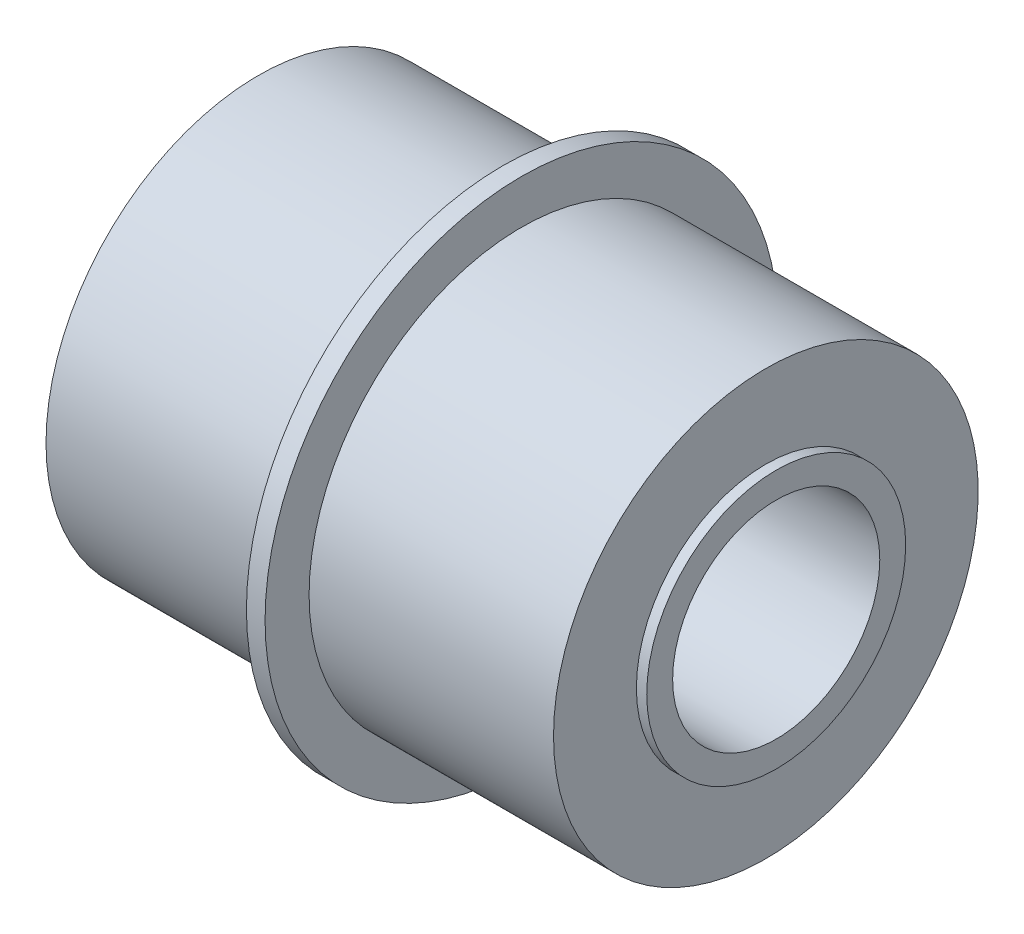
SolidWorks part; units mm, degrees
ref_plane "前视基准面" through (0, 0, 0) normal (0, 0, 1) x (1, 0, 0)
ref_plane "上视基准面" through (0, 0, 0) normal (0, 1, 0) x (1, 0, 0)
ref_plane "右视基准面" through (0, 0, 0) normal (1, 0, 0) x (0, 0, -1)
sketch "草图1" plane through (0, 0, 0) normal (0, 0, 1) x (1, 0, 0)
  line L0 (-73.222, 0) -> (73.222, 0) construction
  line L1 (0, 0) -> (0, 24.75) construction
  line L2 (-0.9, 24.75) -> (0.9, 24.75)
  line L3 (0.9, 24.75) -> (0.9, 20.5)
  line L4 (0.9, 20.5) -> (24.5, 20.5)
  line L5 (24.5, 20.5) -> (24.5, 12.5)
  line L6 (24.5, 12.5) -> (25.5, 12.5)
  line L7 (25.5, 12.5) -> (25.5, 10)
  line L8 (25.5, 10) -> (-25.5, 10)
  line L9 (-25.5, 12.5) -> (-25.5, 10)
  line L10 (-24.5, 12.5) -> (-25.5, 12.5)
  line L11 (-24.5, 20.5) -> (-24.5, 12.5)
  line L12 (-0.9, 20.5) -> (-24.5, 20.5)
  line L13 (-0.9, 24.75) -> (-0.9, 20.5)
  point P13 (0, 10)
  dimension "D1" = 10
  dimension "D2" = 12.5
  dimension "D3" = 20.5
  dimension "D4" = 24.75
  dimension "D5" = 0.9
  dimension "D6" = 24.5
  dimension "D7" = 25.5
revolve "旋转1" add sketch "草图1" angle 360 about L0
